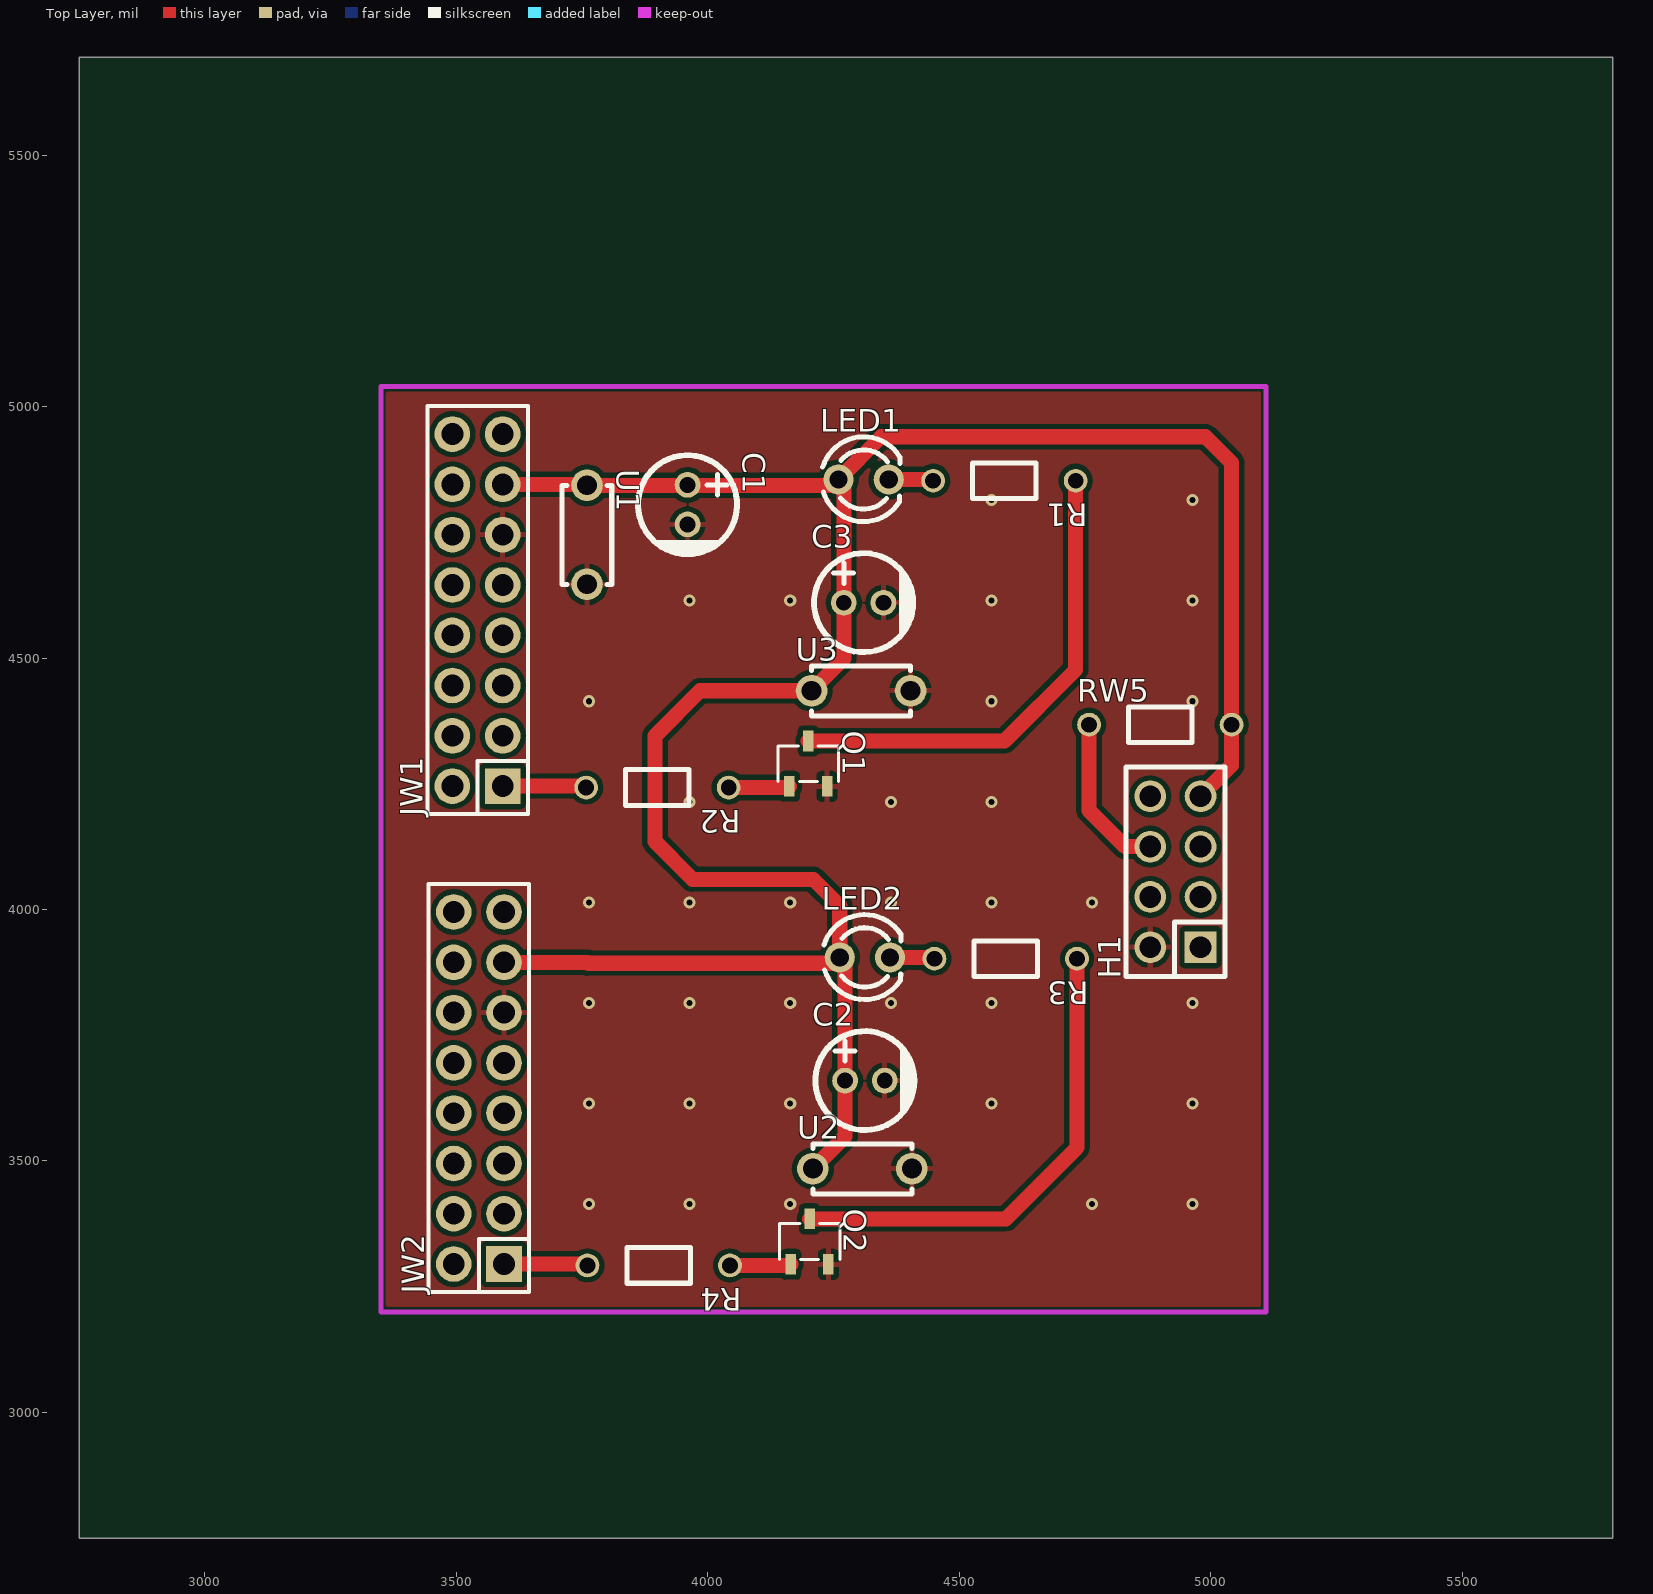
[diagram p0: Top Layer view]
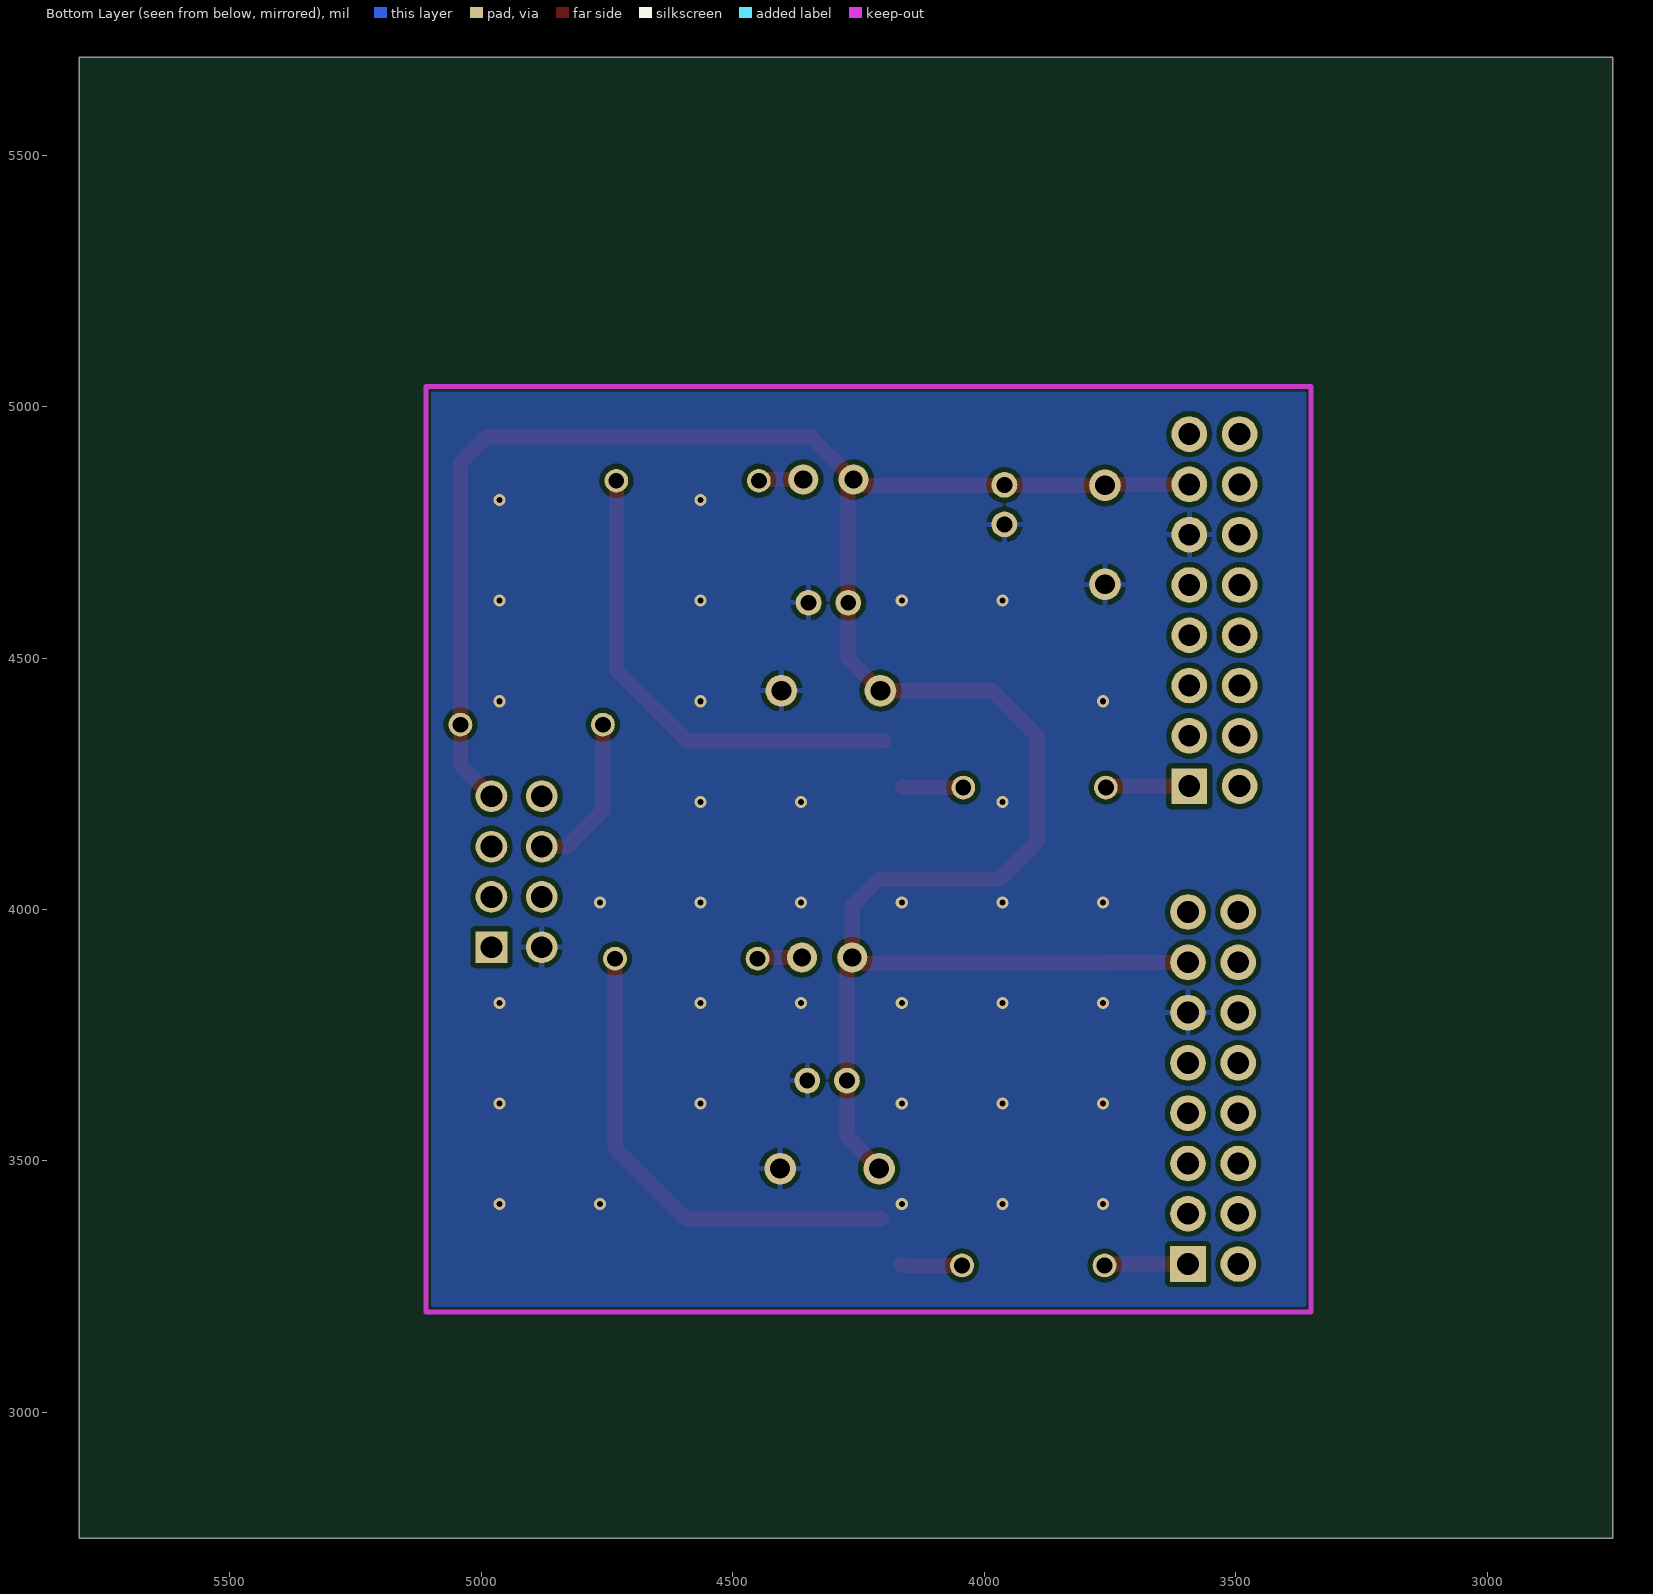
[diagram p1: Bottom Layer view, seen from below]
# Altium PCB MISC82880.pcbdoc
Units mil, origin at the board's own origin, x right, y up, seen from the top; angles counter-clockwise.
Board outline 3050 x 2945 mil, 2 copper layers (Top Layer, Bottom Layer), stack 62.206 mil thick; 18 components, 21 nets, 72 pads, 34 vias.

## Layer stack, top to bottom
Top Solder Mask Layer: solder mask 0.394, Dk 3.3
Top Layer: signal copper 1.379
Dielectric1: surface 59.449, FR4, Dk 4.5
Bottom Layer: signal copper 1.378
Bottom Solder Mask Layer: solder mask 0.394, Dk 3.3

## Board outline
5800,2750 2750,2750 2750,5695 5800,5695

## Design rules (kind name [scope] priority, off if disabled: settings)
BoardOutlineClearance copperThickness2oz_1 [All] p2 off: genericclearance=7.99 ignorepadtopadclearanceinfootprint=FALSE except(0: Arc-SplitContinuation Track-SplitContinuation SMDPad-SplitContinuation THPad-SplitContinuation Via-SplitContinuation Fill-SplitContinuation Region-SplitContinuation Poly-SplitContinuation Text-SplitContinuation Hole-SplitContinuation; 5.98: Arc-CutoutEdge SMDPad-CutoutEdge THPad-CutoutEdge Via-CutoutEdge Fill-CutoutEdge Region-CutoutEdge Text-CutoutEdge; 6.93: Hole-OutlineEdge Hole-CutoutEdge; 10: Poly-OutlineEdge Poly-CutoutEdge; 11.81: Arc-OutlineEdge Track-OutlineEdge SMDPad-OutlineEdge THPad-OutlineEdge Via-OutlineEdge Fill-OutlineEdge Region-OutlineEdge Text-OutlineEdge Track-CutoutEdge)
BoardOutlineClearance copperThickness1oz_1 [All] p4: genericclearance=4.02 ignorepadtopadclearanceinfootprint=FALSE except(0: Arc-SplitContinuation Track-SplitContinuation SMDPad-SplitContinuation THPad-SplitContinuation Via-SplitContinuation Fill-SplitContinuation Region-SplitContinuation Poly-SplitContinuation Text-SplitContinuation Hole-SplitContinuation; 6: SMDPad-CutoutEdge THPad-CutoutEdge Via-CutoutEdge Fill-CutoutEdge Region-CutoutEdge Text-CutoutEdge; 6.93: Hole-OutlineEdge Hole-CutoutEdge; 10: Poly-OutlineEdge Poly-CutoutEdge; 11.8: Arc-OutlineEdge Track-OutlineEdge SMDPad-OutlineEdge THPad-OutlineEdge Via-OutlineEdge Fill-OutlineEdge Region-OutlineEdge Text-OutlineEdge; 11.81: Arc-CutoutEdge Track-CutoutEdge)
Clearance copperThickness2oz [All] p1 off: gap=7.99 ignorepadtopadclearanceinfootprint=FALSE except(5.98: SMDPad-Track SMDPad-SMDPad THPad-Track SMDPad-THPad THPad-THPad Track-Via SMDPad-Via THPad-Via Via-Via Fill-Track Region-Track Fill-SMDPad Region-SMDPad Fill-THPad Region-THPad Fill-Via Region-Via Fill-Fill Fill-Region Region-Region Arc-Track Arc-SMDPad Arc-THPad Arc-Via Fill-Arc Region-Arc Arc-Arc Text-Track SMDPad-Text Text-THPad Text-Via Fill-Text Region-Text Arc-Text Text-Text; 6.93: Hole-Track Hole-SMDPad Hole-THPad Hole-Via Fill-Hole Region-Hole Hole-Arc Hole-Text; 10: Poly-Track Poly-SMDPad Poly-THPad Poly-Via Poly-Fill Poly-Region Poly-Poly Poly-Arc Poly-Text Poly-Hole)
Clearance copperThickness1oz [All] p3: gap=4.02 ignorepadtopadclearanceinfootprint=FALSE except(5.98: SMDPad-Track SMDPad-SMDPad THPad-Track SMDPad-THPad THPad-THPad Track-Via SMDPad-Via THPad-Via Via-Via Fill-Track Region-Track Fill-SMDPad Region-SMDPad Fill-THPad Region-THPad Fill-Via Region-Via Fill-Fill Fill-Region Region-Region; 6: Arc-Track Arc-SMDPad Arc-THPad Arc-Via Fill-Arc Region-Arc Arc-Arc Text-Track SMDPad-Text Text-THPad Text-Via Fill-Text Region-Text Arc-Text Text-Text; 6.93: Hole-Track Hole-SMDPad Hole-THPad Hole-Via Fill-Hole Region-Hole Hole-Arc Hole-Text; 10: Poly-Track Poly-SMDPad Poly-THPad Poly-Via Poly-Fill Poly-Region Poly-Poly Poly-Arc Poly-Text Poly-Hole)
Creepage creepage [All] p1: checkdistance=0 ignoreinternallayers=TRUE applytopolygonpour=TRUE
DiffPairsRouting differentialPair [All] p1: maxlimit=6 minlimit=6 mostfreqgap=6 toplayer_minwidth=5 toplayer_prefwidth=10 toplayer_maxwidth=100 toplayer_mingap=6 toplayer_prefgap=6 toplayer_maxgap=6 bottomlayer_minwidth=5 bottomlayer_prefwidth=10 bottomlayer_maxwidth=100 bottomlayer_mingap=6 bottomlayer_prefgap=6 bottomlayer_maxgap=6 maxuncoupledlength=10
HoleToHoleClearance otherClearance [All] p1: gap=11.81 allowstackedmicrovias=TRUE
Length netLength [All] p1: minlimit=0 maxlimit=0
MatchedLengths netLengthTolerance [All] p1: tolerance=1000
PasteMaskExpansion pasteMaskExpansion [All] p1: expansion=0
PlaneConnect innerPlane [All] p1: planeconnectstyle=Relief reliefexpansion=20 reliefentries=4 reliefconductorwidth=10 reliefairgap=10
PolygonConnect copperRegion [(InNet('GND'))] p1: connectstyle=Relief reliefconductorwidth=10 reliefentries=4 polygonreliefangle="90 Angle" airgapwidth=10 via.connectstyle=Relief via.reliefconductorwidth=10 via.reliefentries=4 via.polygonreliefangle="90 Angle" via.airgapwidth=10
RoutingVias viaSize [All] p1: holewidth=12.01 width=24.02 viastyle="Through Hole" minholewidth=11.81 minwidth=19.68 maxholewidth=248.03 maxwidth=393.7
SolderMaskExpansion solderMaskExpansion [IsVia] p1: expansion=-1000 istentingtop=TRUE
SolderMaskExpansion solderMaskExpansion [All] p2: expansion=2 istentingtop=FALSE
Width copperThickness2oz_2 [All] p1 off: maxlimit=100 minlimit=8 preferedwidth=10
Width copperThickness1oz_2 [All] p2: maxlimit=100 minlimit=5 preferedwidth=10

## Components (designator, comment, footprint, x,y, rotation, side; value= is the part's Value field where it differs from the comment)
C1 "10uF" CAP-TH_BD5.0-P2.00-D0.8-FD-10UF50VC110GL 3960,4805 r270 top
C2 "10uF" CAP-TH_BD5.0-P2.00-D0.8-FD-10UF50VC110GL 4312.62,3659.69 r0 top
C3 "10uF" CAP-TH_BD5.0-P2.00-D0.8-FD-10UF50VC110GL 4310,4610 r0 top
H1 "" HDR-TH_8P-P2.54-V-F-R2-C4-S2.54-1 4930,4075 r90 top
JW1 "" HDR-TH_16P-P2.54-V-F-R2-C8-S2.54-1 3542.38,4595.31 r90 top
JW2 "" HDR-TH_16P-P2.54-V-F-R2-C8-S2.54-1 3545,3645 r90 top
LED1 "" LED_TH-3mm 4310,4855 r0 top
LED2 "" LED_TH-3mm 4312.62,3904.69 r0 top
Q1 "2SC2412KT146Q" SOT-346_L2.9-W1.6-P1.90-LS2.8-TR-CW-1 4200,4290 r270 top
Q2 "2SC2412KT146Q" SOT-346_L2.9-W1.6-P1.90-LS2.8-TR-CW-1 4202.62,3339.69 r270 top
R1 "100Ω" Res_1/8W 4590,4855 r180 top
R2 "100Ω" Res_1/8W 3900,4245 r180 top
R3 "100Ω" Res_1/8W 4592.62,3904.69 r180 top
R4 "100Ω" Res_1/8W 3902.62,3294.69 r180 top
RW5 "4.7kΩ" Res_1/8W 4900,4365 r0 top
U1 "100nF" CAP-TH_L5.0-W2.5-P5.00-D1.0 3760,4745 r270 top
U2 "100nF" CAP-TH_L5.0-W2.5-P5.00-D1.0 4307.62,3484.69 r0 top
U3 "100nF" CAP-TH_L5.0-W2.5-P5.00-D1.0 4305,4435 r0 top

## Footprints (in the part's own frame and the unit in brackets; to place one, negate y for a bottom-side part, rotate by r counter-clockwise, add the part's x,y. Pads: shape width x height; smd on the part's side, far side on the other; paste and mask are expansions set on the pad)
CAP-TH_BD5.0-P2.00-D0.8-FD-10UF50VC110GL [mm]
  round 1.3 hole 0.8: 1(-1,0) 2(1,0)
  silkscreen extent -2.5,-2.5 2.5,2.5
CAP-TH_L5.0-W2.5-P5.00-D1.0 [mm]
  round 1.6 hole 1: 1(-2.5,0) 2(2.5,0)
  silkscreen extent -2.5,-1.27 2.5,1.25
HDR-TH_8P-P2.54-V-F-R2-C4-S2.54-1 [mm]
  rect 1.6x1.6 hole 1.1: 1(-3.81,-1.27)
  round 1.6 hole 1.1: 2(-3.81,1.27) 3(-1.27,-1.27) 4(-1.27,1.27) 5(1.27,-1.27) 6(1.27,1.27) 7(3.81,-1.27) 8(3.81,1.27)
  silkscreen extent -5.28,-2.5 5.28,2.5
HDR-TH_16P-P2.54-V-F-R2-C8-S2.54-1 [mm]
  rect 1.8x1.8 hole 1.1: 1(-8.89,-1.27)
  round 1.8 hole 1.1: 2(-8.89,1.27) 3(-6.35,-1.27) 4(-6.35,1.27) 5(-3.81,-1.27) 6(-3.81,1.27) 7(-1.27,-1.27) 8(-1.27,1.27) 9(1.27,-1.27) 10(1.27,1.27) 11(3.81,-1.27) 12(3.81,1.27) 13(6.35,-1.27) 14(6.35,1.27) 15(8.89,-1.27) 16(8.89,1.27)
  silkscreen extent -10.3,-2.54 10.3,2.54
LED_TH-3mm [mil]
  round 60 hole 36 paste+0 mask+2: 1(-50,0) 2(50,0)
  silkscreen extent -81,-84 72,85
Res_1/8W [mil]
  round 47.2 hole 31.5 paste+0 mask+2: 1(-141.7,2.48) 2(141.7,2.48)
  silkscreen extent -63,-33 63,38
SOT-346_L2.9-W1.6-P1.90-LS2.8-TR-CW-1 [mm]
  rect 1.045x0.532 smd: 1(1.148,0.95) 2(1.148,-0.95) 3(-1.148,0)
  silkscreen extent -0.9,-1.53 0.9,1.53

## Via types
v1: diameter 24.02, hole 12, Top Layer to Bottom Layer, 34 vias

## Nets (pads, with @x,y where several pads share a name; then routed paths per layer and width w, separated by ;. In a path a pad name is that pad's centre, name@x,y a point inside that pad or via, vN(x,y) a via of type N, cw(c..) or ccw(c..) an arc to the next point about the centre after c; other vN are vias at no path point)
$1N21: LED1.2 R1.2 | length 89.3
  Top Layer w30: LED1.2 4445.82,4855 R1.2
$1N22: Q1.3 R1.1 | length 966.1
  Top Layer w30: Q1.3 4590.18,4335.18 4731.7,4476.7 R1.1
$1N23: Q1.2 R2.1 | length 121.9
  Top Layer w30: R2.1 4160.3,4242.52 Q1.2
$1N28: Q2.2 R4.1 | length 121.9
  Top Layer w30: R4.1 4162.92,3292.21 Q2.2
$1N29: Q2.3 R3.1 | length 966.1
  Top Layer w30: Q2.3 4592.8,3384.87 4734.32,3526.39 R3.1
$1N30: LED2.2 R3.2 | length 89.3
  Top Layer w30: LED2.2 4448.44,3904.69 R3.2
$1N39: H1.6 RW5.1 | length 322.2
  Top Layer w30: RW5.1 4758.3,4196.7 4830,4125 H1.6
+3.3V: C1.1 C2.1 C3.1 H1.7 JW1.13 JW2.13 LED1.1 LED2.1 RW5.2 U1.1 U2.1 U3.1 | length 4857.5
  Top Layer w30: JW1.13 3758.11,4845.31 U1.1 4248.43,4843.43 LED1.1 ; JW2.13 3760.73,3895 3762.62,3893.11 4251.04,3893.11 LED2.1 ; U2.1 4273.25,3548.74 C2.1 4273.25,3894.06 LED2.1 ; H1.7 5041.7,4286.7 RW5.2 5041.7,4888.3 4990,4940 4345,4940 LED1.1 ; LED1.1 4270.63,4844.37 C3.1 4270.63,4499.06 U3.1 3985,4435 3895,4345 3895,4135 3970,4060 4210,4060 4262.62,4007.38 LED2.1
BAT3V: H1.8
GND: C1.2 C2.2 C3.2 H1.2 JW1.11 JW2.11 Q1.1 Q2.1 U1.2 U2.2 U3.2
  other v1: 3764.1,3414.1 3964.1,3414.1 4164.1,3414.1 4764.1,3414.1 4964.1,3414.1 3764.1,3614.1 3964.1,3614.1 4164.1,3614.1 4564.1,3614.1 4964.1,3614.1 3764.1,3814.1 3964.1,3814.1 4164.1,3814.1 4364.1,3814.1 4564.1,3814.1 4964.1,3814.1 3764.1,4014.1 3964.1,4014.1 4164.1,4014.1 4364.1,4014.1 4564.1,4014.1 4764.1,4014.1 3964.1,4214.1 4364.1,4214.1 4564.1,4214.1 3764.1,4414.1 4564.1,4414.1 4964.1,4414.1 3964.1,4614.1 4164.1,4614.1 4564.1,4614.1 4964.1,4614.1 4564.1,4814.1 4964.1,4814.1
PPS: H1.4
RXD1: JW1.7
RXD2: JW2.7
RXD3: H1.1
STATE_LED1: JW1.1 R2.2 | length 167.1
  Top Layer w30: JW1.1 3755.51,4245.31 R2.2
STATE_LED2: JW2.1 R4.2 | length 167.1
  Top Layer w30: JW2.1 3758.13,3295 R4.2
TXD1: JW1.5
TXD2: JW2.5
TXD3: H1.3
WIR_RST1: JW1.9
WIR_RST2: JW2.9
pads on no net: H1.5 JW1.2 JW1.3 JW1.4 JW1.6 JW1.8 JW1.10 JW1.12 JW1.14 JW1.15 JW1.16 JW2.2 JW2.3 JW2.4 JW2.6 JW2.8 JW2.10 JW2.12 JW2.14 JW2.15 JW2.16

## Polygon pours and split planes (outlines as drawn)
GND on Top Layer (solid, remove dead copper, pour order 0): 3000,5445 3000,3000 5510,3000 5510,5445
GND on Bottom Layer (solid, remove dead copper, pour order 2): 3035,5220 3035,3100 5550,3100 5550,5220

## Keep-outs
Board Outline Layer:
  lines w10: 3350,3200 3350,5040 5110,5040 5110,3200 3350,3200